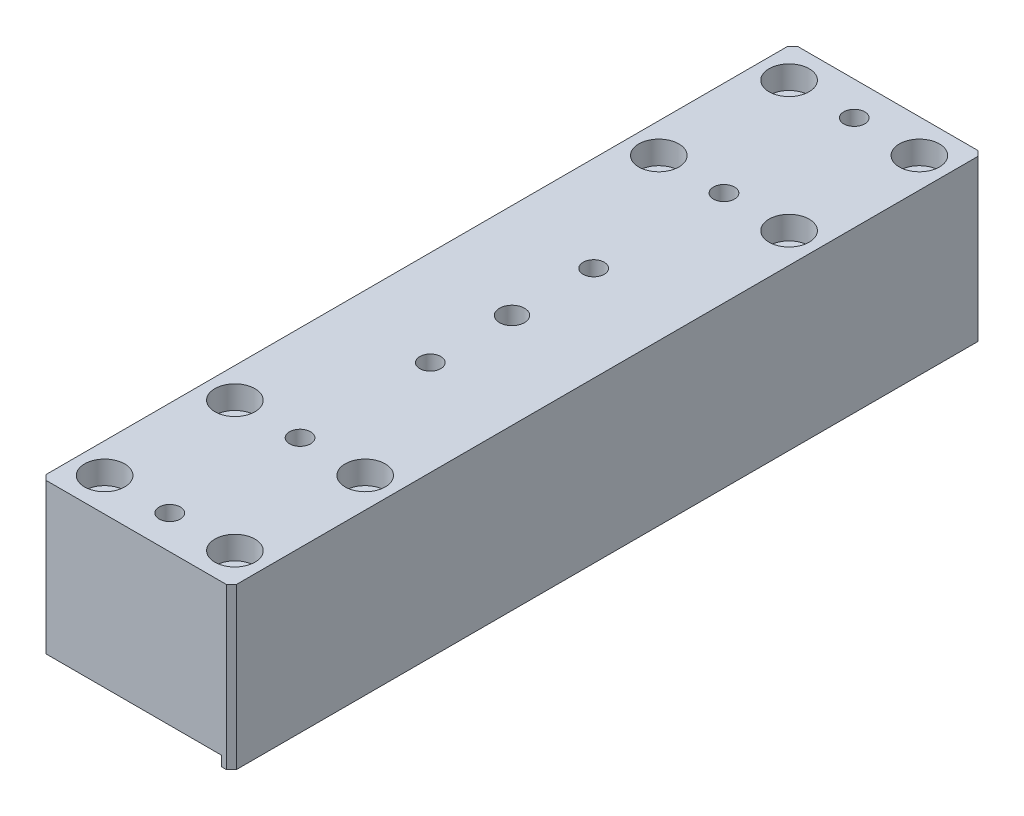
SolidWorks part; units mm, degrees
material "AL6061"
ref_plane "Front View" through (0, 0, 0) normal (0, 0, 1) x (1, 0, 0)
ref_plane "Top View" through (0, 0, 0) normal (0, 1, 0) x (1, 0, 0)
ref_plane "Right View" through (0, 0, 0) normal (1, 0, 0) x (0, 0, -1)
sketch "Sketch1" plane through (0, 0, 0) normal (0, 0, 1) x (1, 0, 0)
  line L0 (0, 0) -> (0, 32)
  line L1 (0, 32) -> (-38, 32)
  line L2 (-38, 32) -> (-38, 2)
  line L3 (-38, 2) -> (-2, 2)
  line L4 (-2, 2) -> (-2, 0)
  line L5 (-2, 0) -> (0, 0)
  dimension "D1" = 30
  dimension "D2" = 38
  dimension "D3" = 2
  dimension "D4" = 2
extrude "Boss-Extrude1" add sketch "Sketch1" along normal mid plane 150
hole_wizard "Hole Size (by socket head cap screw type)1" positions "Sketch2" profile "Sketch3" counterbore size "M4" standard "GB" end condition through all
sketch "Sketch2" plane through (0, 32, 0) normal (0, 1, 0) x (1, 0, 0)
  line L0 (0, 0) -> (-52.7578, 0) construction
  line L4 (-32, 68.3) -> (-6, 68.3)
  line L5 (-32, 68.3) -> (-32, 42.3)
  line L6 (-32, 42.3) -> (-6, 42.3)
  line L7 (-6, 68.3) -> (-6, 42.3)
  line L8 (-6, -68.3) -> (-6, -42.3)
  line L9 (-32, -42.3) -> (-6, -42.3)
  line L10 (-32, -68.3) -> (-32, -42.3)
  line L11 (-32, -68.3) -> (-6, -68.3)
  line L12 (-2, -75) -> (-2, 75) construction
  point P8 (-32, 68.3)
  point P9 (-6, 42.3)
  point P170 (-32, 42.3)
  point P171 (-6, 68.3)
  point P172 (-6, -68.3)
  point P173 (-6, -42.3)
  point P174 (-32, -42.3)
  point P175 (-32, -68.3)
  dimension "D1" = 110.6
  dimension "D2" = 26
  dimension "D3" = 4
sketch "Sketch3" plane through (-32, 32, 68.3) normal (1, 0, 0) x (0, 0, 1)
  line L0 (0, 0) -> (0, 32)
  line L1 (0, 32) -> (2.25, 32)
  line L3 (2.25, 32) -> (2.25, 4.6)
  line L4 (2.25, 4.6) -> (4, 4.6)
  line L5 (4, 4.6) -> (4, 0)
  line L7 (4, 0) -> (0, 0)
  line L11 (0, -6.35) -> (0, 107.95) construction
  dimension "通孔孔直径" = 4.5
  dimension "通孔孔深度" = 32
  dimension "柱形沉头孔直径" = 8
  dimension "柱形沉头孔深度" = 4.6
hole_wizard "M5 Tapped Hole1" positions "Sketch4" profile "Sketch5" tap size "M5" standard "GB"
sketch "Sketch4" plane through (-38, 0, 0) normal (1, 0, 0) x (0, 0, -1)
  line L0 (0, 0) -> (0, 30.7571) construction
  line L3 (-78.5654, 17) -> (85.5113, 17) construction
  line L4 (-75, 32) -> (75, 32) construction
  point P13 (-20, 17)
  point P16 (20, 17)
  point P17 (0, 17)
  dimension "D1" = 40
  dimension "D2" = 15
sketch "Sketch5" plane through (-38, 17, 0) normal (0, 1, 0) x (0, 0, 1)
  line L0 (0, 0) -> (0, 13.6618)
  line L1 (0, 13.6618) -> (2.1, 12.4)
  line L2 (2.1, 12.4) -> (2.1, 0)
  line L5 (2.1, 0) -> (0, 0)
  line L10 (0, 13.6618) -> (-2.1, 12.4) construction
  line L11 (0, -6.35) -> (0, 107.95) construction
  dimension "螺纹孔钻头直径" = 4.2
  dimension "螺纹孔钻头深度" = 12.4
  dimension "导头角度" = 118
cosmetic thread "Hole Thread1" parameters "D1"=10, "D2"=5
cosmetic thread "Hole Thread2" parameters "D1"=10, "D2"=5
cosmetic thread "Hole Thread3" parameters "D1"=10, "D2"=5
hole_wizard "M5 Tapped Hole2" positions "Sketch8" profile "Sketch9" tap size "M5" standard "GB"
sketch "Sketch8" plane through (0, 32, 0) normal (0, 1, 0) x (1, 0, 0)
  line L0 (0, 0) -> (-54.3558, 0) construction
  line L3 (-19, 75) -> (-19, -82.8964) construction
  line L4 (0, 75) -> (-38, 75) construction
  line L5 (-32, 68.3) -> (-6, 68.3) construction
  line L8 (-32, 42.3) -> (-6, 42.3) construction
  point P15 (-19, 68.3)
  point P17 (-19, 42.3)
  point P22 (-19, -42.3)
  point P23 (-19, -68.3)
  point P46 (-19, 16.3)
  point P49 (-19, -16.3)
  dimension "D1" = 26
sketch "Sketch9" plane through (-19, 32, 16.3) normal (1, 0, 0) x (0, 0, 1)
  line L0 (0, 0) -> (0, 13.6618)
  line L1 (0, 13.6618) -> (2.1, 12.4)
  line L2 (2.1, 12.4) -> (2.1, 0)
  line L5 (2.1, 0) -> (0, 0)
  line L10 (0, 13.6618) -> (-2.1, 12.4) construction
  line L11 (0, -6.35) -> (0, 107.95) construction
  dimension "螺纹孔钻头直径" = 4.2
  dimension "螺纹孔钻头深度" = 12.4
  dimension "导头角度" = 118
cosmetic thread "Hole Thread4" parameters "D1"=10, "D2"=5
cosmetic thread "Hole Thread5" parameters "D1"=10, "D2"=5
cosmetic thread "Hole Thread6" parameters "D1"=10, "D2"=5
cosmetic thread "Hole Thread7" parameters "D1"=10, "D2"=5
cosmetic thread "Hole Thread8" parameters "D1"=10, "D2"=5
cosmetic thread "Hole Thread9" parameters "D1"=10, "D2"=5
chamfer "Chamfer1" distance 1 angle 45 4 edges at (0, 16, 75) (-38, 17, 75) (-38, 17, -75) (0, 16, -75)
hole_wizard "Size mm Blind Pin Hole1" positions "Sketch10" profile "Sketch11" hole size "Ø5.0" standard "GB"
sketch "Sketch10" plane through (0, 32, 0) normal (0, 1, 0) x (1, 0, 0)
  line L0 (-19, 16.3) -> (-19, -16.3) construction
  point P9 (-19, 0)
sketch "Sketch11" plane through (-19, 32, 0) normal (1, 0, 0) x (0, 0, 1)
  line L0 (0, 0) -> (0, 9.0022)
  line L1 (0, 9.0022) -> (2.5, 7.5)
  line L2 (2.5, 7.5) -> (2.5, 0)
  line L5 (2.5, 0) -> (0, 0)
  line L10 (0, 9.0022) -> (-2.5, 7.5) construction
  line L11 (0, -6.35) -> (0, 107.95) construction
  dimension "孔直径" = 5
  dimension "孔深度" = 7.5
  dimension "导头角度" = 118
